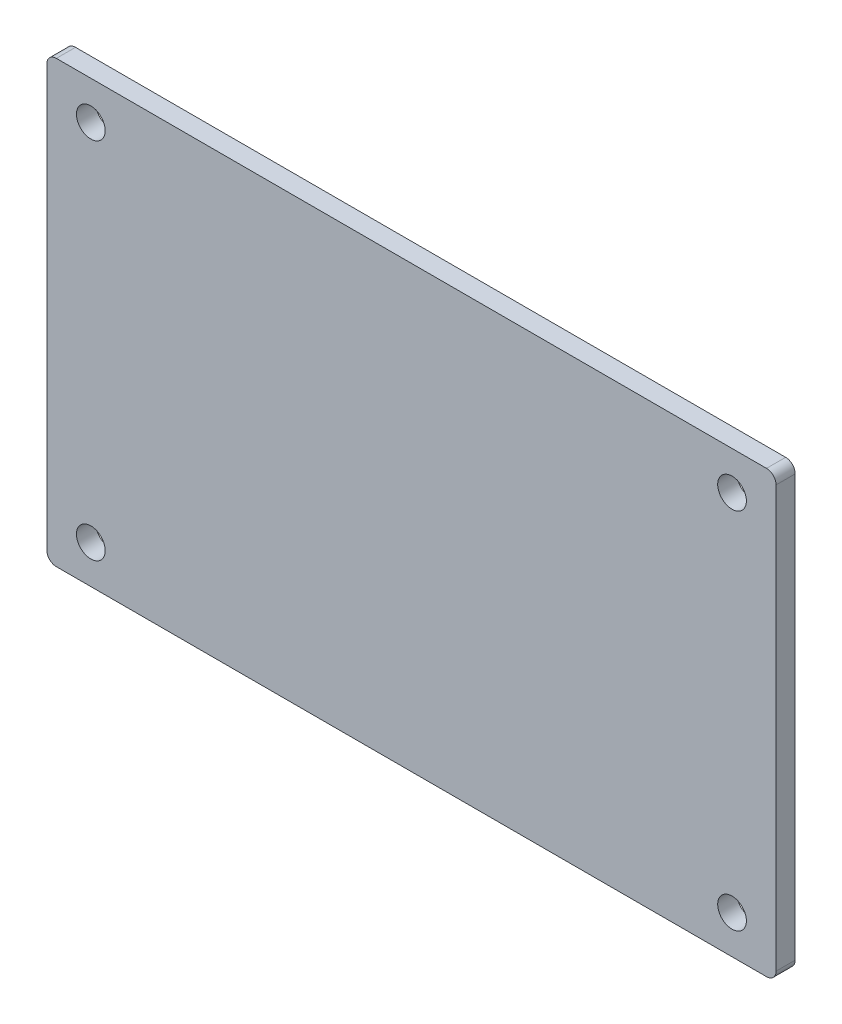
SolidWorks part; units mm, degrees
material "Q235B"
ref_plane "Front Plane" through (0, 0, 0) normal (0, 0, 1) x (1, 0, 0)
ref_plane "Top Plane" through (0, 0, 0) normal (0, 1, 0) x (1, 0, 0)
ref_plane "Right Plane" through (0, 0, 0) normal (1, 0, 0) x (0, 0, -1)
sketch "Sketch1" plane through (0, 0, 0) normal (0, 0, 1) x (1, 0, 0)
  line L1 (190.5, -115) -> (-190.5, -115)
  line L2 (190.5, -115) -> (190.5, 115)
  line L3 (190.5, 115) -> (-190.5, 115)
  line L4 (-190.5, -115) -> (-190.5, 115)
  line L5 (190.5, -115) -> (-190.5, 115) construction
  line L6 (190.5, 115) -> (-190.5, -115) construction
  point P0 (0, 0)
  dimension "D1" = 230
  dimension "D2" = 381
extrude "Boss-Extrude1" add sketch "Sketch1" along normal mid plane 10
hole_wizard "Ø15 Hole1" positions "Sketch2" profile "Sketch3" hole size "Ø15.0" standard "GB" end condition up to next
sketch "Sketch2" plane through (0, 0, 5) normal (0, 0, 1) x (1, 0, 0)
  line L0 (0, 115) -> (0, 0) construction
  line L1 (190.5, 115) -> (-190.5, 115) construction
  line L2 (0, 0) -> (-190.5, 0) construction
  line L3 (-190.5, 115) -> (-190.5, -115) construction
  point P0 (-167.5, 95)
  point P13 (167.5, 95)
  point P14 (167.5, -95)
  point P15 (-167.5, -95)
  dimension "D1" = 335
  dimension "D2" = 190
sketch "Sketch3" plane through (-167.5, 95, 5) normal (1, 0, 0) x (0, -1, 0)
  line L0 (0, 0) -> (0, 10)
  line L1 (0, 10) -> (7.5, 10)
  line L2 (7.5, 10) -> (7.5, 0)
  line L5 (7.5, 0) -> (0, 0)
  line L11 (0, -6.35) -> (0, 107.95) construction
  dimension "通孔孔直径" = 15
  dimension "通孔孔深度" = 10
chamfer "Chamfer1" [suppressed] distance 10 angle 45
fillet "Fillet2" radius 5 4 edges at (190.5, 115, 0) (190.5, -115, 0) (-190.5, -115, 0) (-190.5, 115, 0)
